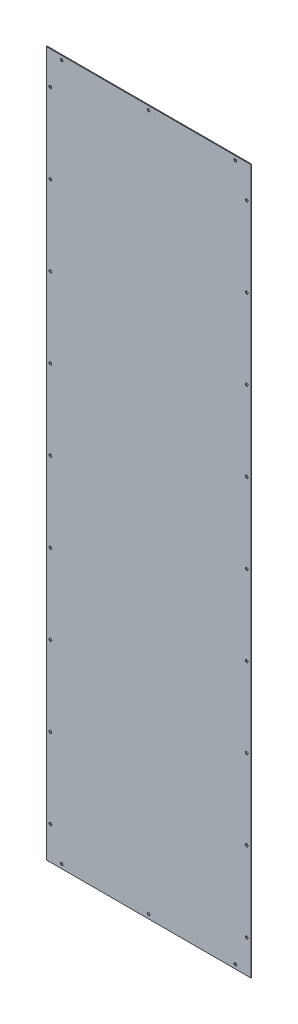
SolidWorks part; units mm, degrees
material "304"
ref_plane "前视基准面" through (0, 0, 0) normal (0, 0, 1) x (1, 0, 0)
ref_plane "上视基准面" through (0, 0, 0) normal (0, 1, 0) x (1, 0, 0)
ref_plane "右视基准面" through (0, 0, 0) normal (1, 0, 0) x (0, 0, -1)
sketch "草图1" plane through (0, 0, 0) normal (0, 0, 1) x (1, 0, 0)
  line L0 (0, 0) -> (451.2544, 0) construction
  line L1 (-247.25, 851.5) -> (247.25, 851.5)
  line L2 (-247.25, 851.5) -> (-247.25, -851.5)
  line L3 (-247.25, -851.5) -> (247.25, -851.5)
  line L4 (247.25, 851.5) -> (247.25, -851.5)
  line L5 (-247.25, 851.5) -> (247.25, -851.5) construction
  line L6 (-247.25, -851.5) -> (247.25, 851.5) construction
  line L7 (0, 0) -> (0, 412.8629) construction
  circle A0 centre (-237.25, 0) radius 3.25
  circle A1 centre (-237.25, -192.875) radius 3.25
  circle A2 centre (-237.25, -385.75) radius 3.25
  circle A3 centre (-237.25, -578.625) radius 3.25
  circle A4 centre (-237.25, -771.5) radius 3.25
  circle A34 centre (0, -841.5) radius 3.25
  circle A35 centre (0, 841.5) radius 3.25
  circle A36 centre (-237.25, 771.5) radius 3.25
  circle A37 centre (-237.25, 578.625) radius 3.25
  circle A38 centre (-237.25, 385.75) radius 3.25
  circle A39 centre (-237.25, 192.875) radius 3.25
  circle A40 centre (237.25, 192.875) radius 3.25
  circle A41 centre (237.25, 385.75) radius 3.25
  circle A42 centre (237.25, 578.625) radius 3.25
  circle A43 centre (237.25, 771.5) radius 3.25
  circle A44 centre (237.25, -771.5) radius 3.25
  circle A45 centre (237.25, -578.625) radius 3.25
  circle A46 centre (237.25, -385.75) radius 3.25
  circle A47 centre (237.25, -192.875) radius 3.25
  circle A48 centre (237.25, 0) radius 3.25
  circle A49 centre (-210, 841.5) radius 3.25
  circle A50 centre (210, 841.5) radius 3.25
  circle A51 centre (-210, -841.5) radius 3.25
  circle A52 centre (210, -841.5) radius 3.25
  point P0 (0, 0)
  dimension "D3" = 6.5
  dimension "D8" = 420
  dimension "D1" = 494.5
  dimension "D2" = 1703
  dimension "D4" = 10
  dimension "D6" = 10
  dimension "D7" = 80
  dimension "D5" = 5
extrude "凸台-拉伸1" add sketch "草图1" along normal blind 2
sketch "草图2" plane through (0, -851.5, 0) normal (0, -1, 0) x (-1, 0, 0)
  line L0 (247.25, 0) -> (-247.25, 0) construction
  line L1 (-247.25, -2) -> (-244.75, -2)
  line L2 (-247.25, -2) -> (-247.25, 0)
  line L3 (-247.25, 0) -> (-244.75, 0)
  line L4 (-244.75, -2) -> (-244.75, 0)
  dimension "D1" = 2.5
